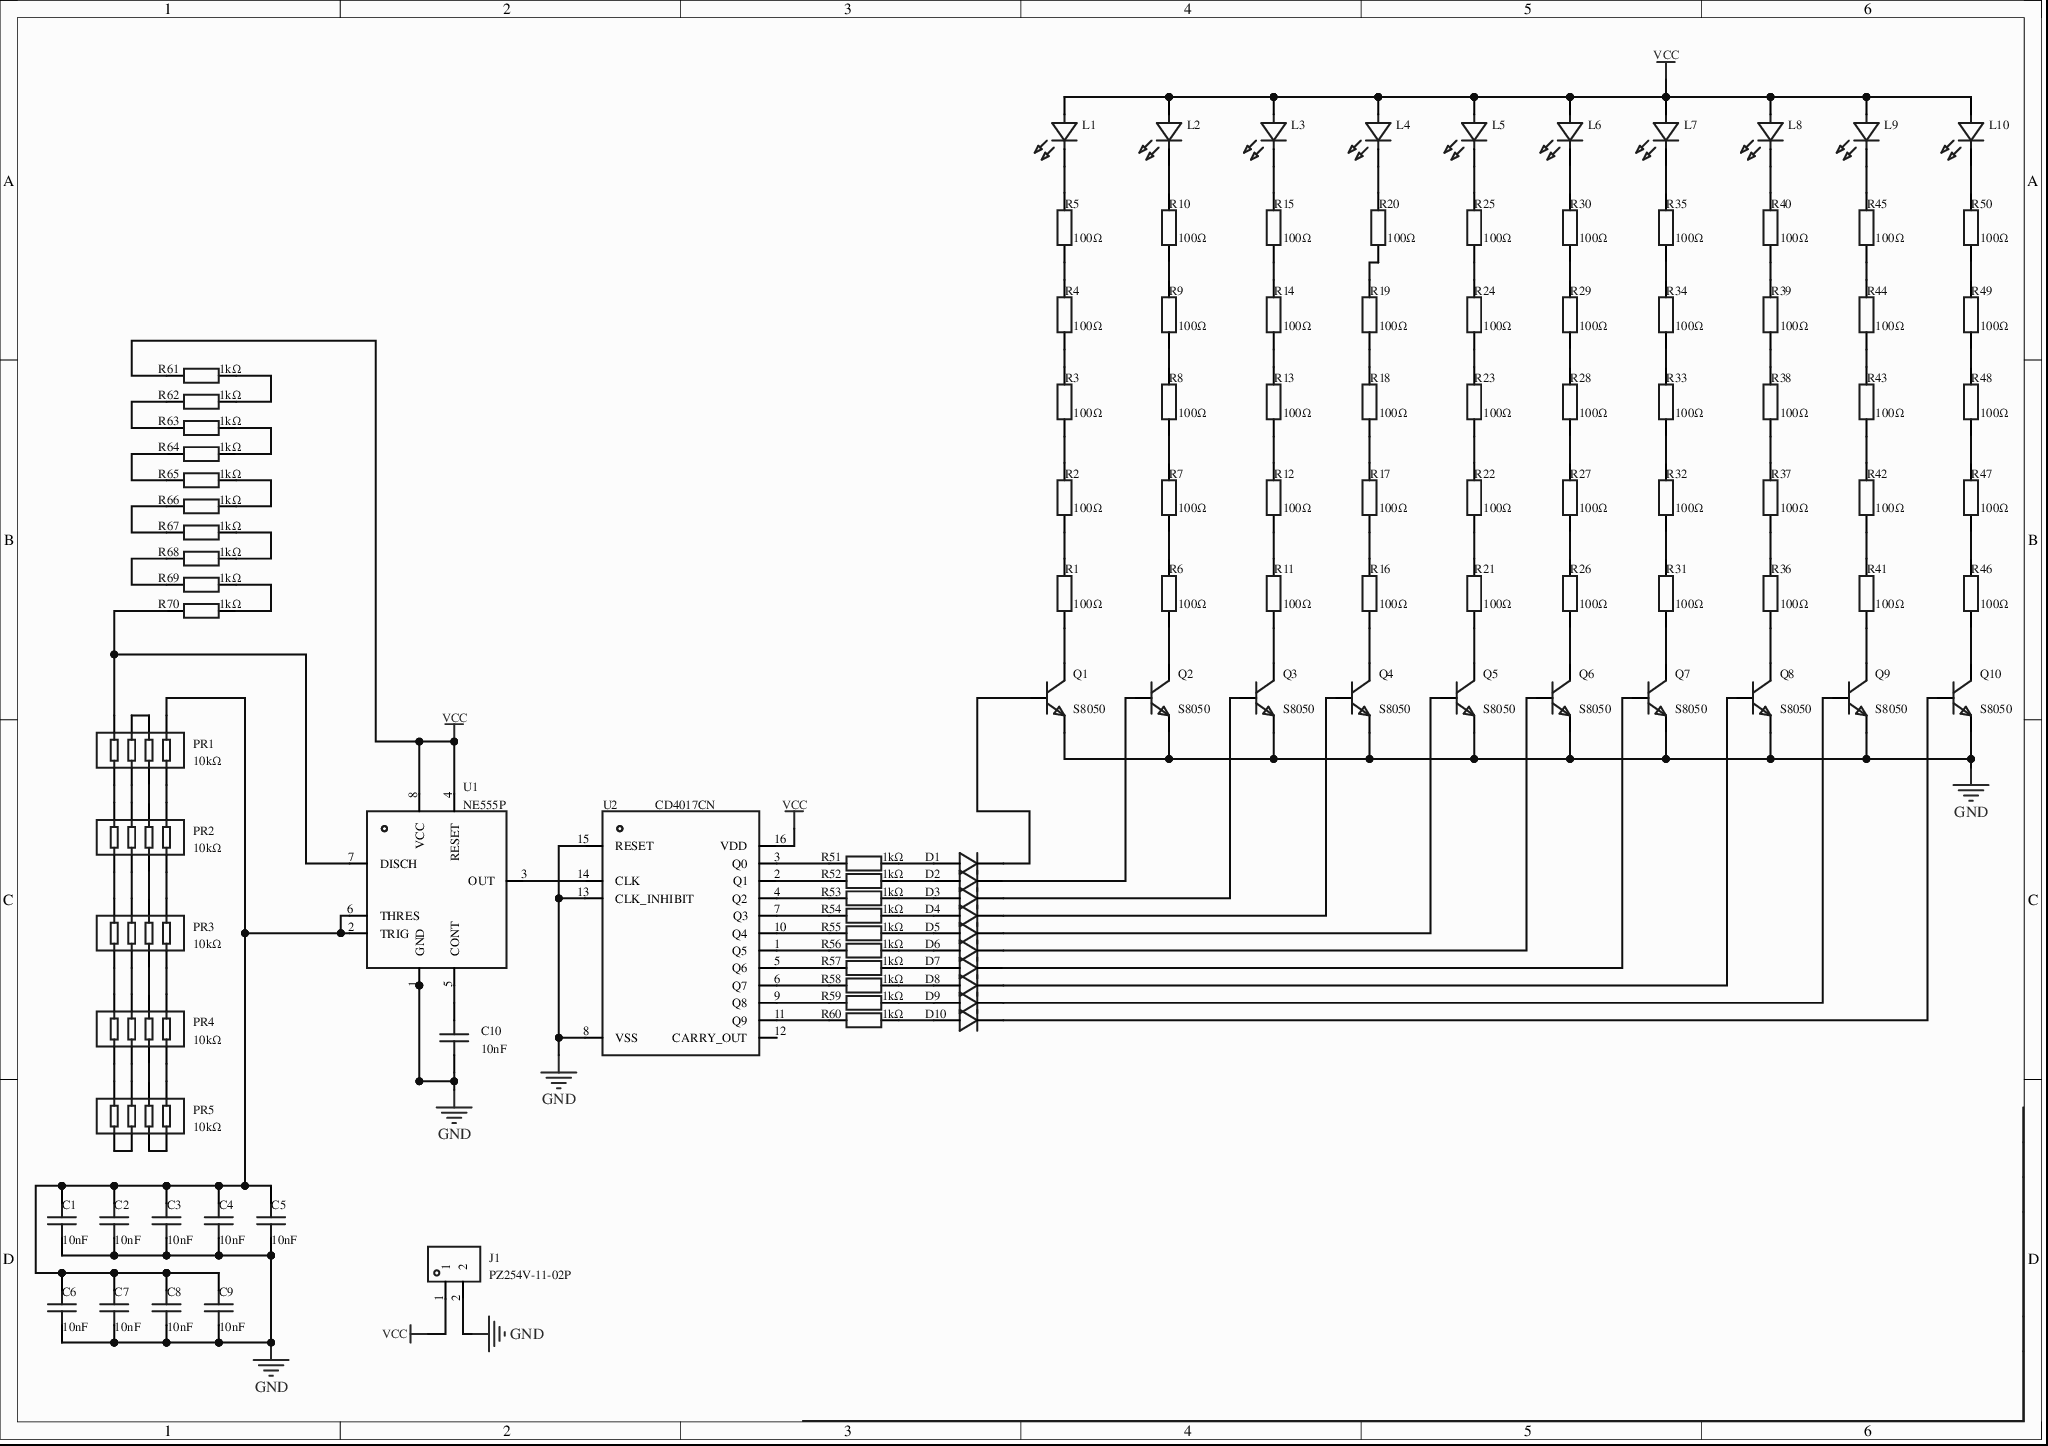
[diagram p0: MISC51825-3.schdoc]
# Altium project MISC51825-2.PrjPcb
1 sheet, 118 parts. Net scope: global (net labels, ports and power ports of the same name join across sheets).
Board file: MISC51825.pcbdoc

## Sheet MISC51825-3.schdoc
size 297 x 209 mm; Version: V1.0; @Project Name: MISC51825; @Page Count: 1; @Update Date: 2026-04-22; @Create Date: 2026-04-22; @Schematic Name: MISC51825; @Page No: 1; @Board Name: MISC51825; @Create Time: 14:32:28; @Update Time: 14:38:12; Size: A4

### Parts
C1  10nF  [CAP-TH_L8.0-W2.8-P5.08-D0.6]
C2  10nF  [CAP-TH_L8.0-W2.8-P5.08-D0.6]
C3  10nF  [CAP-TH_L8.0-W2.8-P5.08-D0.6]
C4  10nF  [CAP-TH_L8.0-W2.8-P5.08-D0.6]
C5  10nF  [CAP-TH_L8.0-W2.8-P5.08-D0.6]
C6  10nF  [CAP-TH_L8.0-W2.8-P5.08-D0.6]
C7  10nF  [CAP-TH_L8.0-W2.8-P5.08-D0.6]
C8  10nF  [CAP-TH_L8.0-W2.8-P5.08-D0.6]
C9  10nF  [CAP-TH_L8.0-W2.8-P5.08-D0.6]
C10  10nF  [CAP-TH_L8.0-W2.8-P5.08-D0.6]
D1  1N4148TR  [DO-35_BD2.0-L4.2-P8.20-D0.5-RD]  (value not drawn)
D2  1N4148TR  [DO-35_BD2.0-L4.2-P8.20-D0.5-RD]  (value not drawn)
D3  1N4148TR  [DO-35_BD2.0-L4.2-P8.20-D0.5-RD]  (value not drawn)
D4  1N4148TR  [DO-35_BD2.0-L4.2-P8.20-D0.5-RD]  (value not drawn)
D5  1N4148TR  [DO-35_BD2.0-L4.2-P8.20-D0.5-RD]  (value not drawn)
D6  1N4148TR  [DO-35_BD2.0-L4.2-P8.20-D0.5-RD]  (value not drawn)
D7  1N4148TR  [DO-35_BD2.0-L4.2-P8.20-D0.5-RD]  (value not drawn)
D8  1N4148TR  [DO-35_BD2.0-L4.2-P8.20-D0.5-RD]  (value not drawn)
D9  1N4148TR  [DO-35_BD2.0-L4.2-P8.20-D0.5-RD]  (value not drawn)
D10  1N4148TR  [DO-35_BD2.0-L4.2-P8.20-D0.5-RD]  (value not drawn)
J1  PZ254V-11-02P  [HDR-TH_2P-P2.54-V-M]
L1  XL-502SURD  [LED-TH_BD5.9-P2.54-RD_RED]  (value not drawn)
L2  XL-502SURD  [LED-TH_BD5.9-P2.54-RD_RED]  (value not drawn)
L3  XL-502SURD  [LED-TH_BD5.9-P2.54-RD_RED]  (value not drawn)
L4  XL-502SURD  [LED-TH_BD5.9-P2.54-RD_RED]  (value not drawn)
L5  XL-502SURD  [LED-TH_BD5.9-P2.54-RD_RED]  (value not drawn)
L6  XL-502SURD  [LED-TH_BD5.9-P2.54-RD_RED]  (value not drawn)
L7  XL-502SURD  [LED-TH_BD5.9-P2.54-RD_RED]  (value not drawn)
L8  XL-502SURD  [LED-TH_BD5.9-P2.54-RD_RED]  (value not drawn)
L9  XL-502SURD  [LED-TH_BD5.9-P2.54-RD_RED]  (value not drawn)
L10  XL-502SURD  [LED-TH_BD5.9-P2.54-RD_RED]  (value not drawn)
PR1  10kΩ  [RES-ARRAY-TH_8P-L20.3-W2.5-P2.54]
PR2  10kΩ  [RES-ARRAY-TH_8P-L20.3-W2.5-P2.54]
PR3  10kΩ  [RES-ARRAY-TH_8P-L20.3-W2.5-P2.54]
PR4  10kΩ  [RES-ARRAY-TH_8P-L20.3-W2.5-P2.54]
PR5  10kΩ  [RES-ARRAY-TH_8P-L20.3-W2.5-P2.54]
Q1  S8050  [TO-92-3_L4.5-W3.5-P1.27-L]
Q2  S8050  [TO-92-3_L4.5-W3.5-P1.27-L]
Q3  S8050  [TO-92-3_L4.5-W3.5-P1.27-L]
Q4  S8050  [TO-92-3_L4.5-W3.5-P1.27-L]
Q5  S8050  [TO-92-3_L4.5-W3.5-P1.27-L]
Q6  S8050  [TO-92-3_L4.5-W3.5-P1.27-L]
Q7  S8050  [TO-92-3_L4.5-W3.5-P1.27-L]
Q8  S8050  [TO-92-3_L4.5-W3.5-P1.27-L]
Q9  S8050  [TO-92-3_L4.5-W3.5-P1.27-L]
Q10  S8050  [TO-92-3_L4.5-W3.5-P1.27-L]
R1  100Ω  [RES-TH_BD2.2-L6.5-P10.50-D0.6]
R2  100Ω  [RES-TH_BD2.2-L6.5-P10.50-D0.6]
R3  100Ω  [RES-TH_BD2.2-L6.5-P10.50-D0.6]
R4  100Ω  [RES-TH_BD2.2-L6.5-P10.50-D0.6]
R5  100Ω  [RES-TH_BD2.2-L6.5-P10.50-D0.6]
R6  100Ω  [RES-TH_BD2.2-L6.5-P10.50-D0.6]
R7  100Ω  [RES-TH_BD2.2-L6.5-P10.50-D0.6]
R8  100Ω  [RES-TH_BD2.2-L6.5-P10.50-D0.6]
R9  100Ω  [RES-TH_BD2.2-L6.5-P10.50-D0.6]
R10  100Ω  [RES-TH_BD2.2-L6.5-P10.50-D0.6]
R11  100Ω  [RES-TH_BD2.2-L6.5-P10.50-D0.6]
R12  100Ω  [RES-TH_BD2.2-L6.5-P10.50-D0.6]
R13  100Ω  [RES-TH_BD2.2-L6.5-P10.50-D0.6]
R14  100Ω  [RES-TH_BD2.2-L6.5-P10.50-D0.6]
R15  100Ω  [RES-TH_BD2.2-L6.5-P10.50-D0.6]
R16  100Ω  [RES-TH_BD2.2-L6.5-P10.50-D0.6]
R17  100Ω  [RES-TH_BD2.2-L6.5-P10.50-D0.6]
R18  100Ω  [RES-TH_BD2.2-L6.5-P10.50-D0.6]
R19  100Ω  [RES-TH_BD2.2-L6.5-P10.50-D0.6]
R20  100Ω  [RES-TH_BD2.2-L6.5-P10.50-D0.6]
R21  100Ω  [RES-TH_BD2.2-L6.5-P10.50-D0.6]
R22  100Ω  [RES-TH_BD2.2-L6.5-P10.50-D0.6]
R23  100Ω  [RES-TH_BD2.2-L6.5-P10.50-D0.6]
R24  100Ω  [RES-TH_BD2.2-L6.5-P10.50-D0.6]
R25  100Ω  [RES-TH_BD2.2-L6.5-P10.50-D0.6]
R26  100Ω  [RES-TH_BD2.2-L6.5-P10.50-D0.6]
R27  100Ω  [RES-TH_BD2.2-L6.5-P10.50-D0.6]
R28  100Ω  [RES-TH_BD2.2-L6.5-P10.50-D0.6]
R29  100Ω  [RES-TH_BD2.2-L6.5-P10.50-D0.6]
R30  100Ω  [RES-TH_BD2.2-L6.5-P10.50-D0.6]
R31  100Ω  [RES-TH_BD2.2-L6.5-P10.50-D0.6]
R32  100Ω  [RES-TH_BD2.2-L6.5-P10.50-D0.6]
R33  100Ω  [RES-TH_BD2.2-L6.5-P10.50-D0.6]
R34  100Ω  [RES-TH_BD2.2-L6.5-P10.50-D0.6]
R35  100Ω  [RES-TH_BD2.2-L6.5-P10.50-D0.6]
R36  100Ω  [RES-TH_BD2.2-L6.5-P10.50-D0.6]
R37  100Ω  [RES-TH_BD2.2-L6.5-P10.50-D0.6]
R38  100Ω  [RES-TH_BD2.2-L6.5-P10.50-D0.6]
R39  100Ω  [RES-TH_BD2.2-L6.5-P10.50-D0.6]
R40  100Ω  [RES-TH_BD2.2-L6.5-P10.50-D0.6]
R41  100Ω  [RES-TH_BD2.2-L6.5-P10.50-D0.6]
R42  100Ω  [RES-TH_BD2.2-L6.5-P10.50-D0.6]
R43  100Ω  [RES-TH_BD2.2-L6.5-P10.50-D0.6]
R44  100Ω  [RES-TH_BD2.2-L6.5-P10.50-D0.6]
R45  100Ω  [RES-TH_BD2.2-L6.5-P10.50-D0.6]
R46  100Ω  [RES-TH_BD2.2-L6.5-P10.50-D0.6]
R47  100Ω  [RES-TH_BD2.2-L6.5-P10.50-D0.6]
R48  100Ω  [RES-TH_BD2.2-L6.5-P10.50-D0.6]
R49  100Ω  [RES-TH_BD2.2-L6.5-P10.50-D0.6]
R50  100Ω  [RES-TH_BD2.2-L6.5-P10.50-D0.6]
R51  1kΩ  [RES-TH_BD2.5-L6.5-P10.50-D0.6]
R52  1kΩ  [RES-TH_BD2.5-L6.5-P10.50-D0.6]
R53  1kΩ  [RES-TH_BD2.5-L6.5-P10.50-D0.6]
R54  1kΩ  [RES-TH_BD2.5-L6.5-P10.50-D0.6]
R55  1kΩ  [RES-TH_BD2.5-L6.5-P10.50-D0.6]
R56  1kΩ  [RES-TH_BD2.5-L6.5-P10.50-D0.6]
R57  1kΩ  [RES-TH_BD2.5-L6.5-P10.50-D0.6]
R58  1kΩ  [RES-TH_BD2.5-L6.5-P10.50-D0.6]
R59  1kΩ  [RES-TH_BD2.5-L6.5-P10.50-D0.6]
R60  1kΩ  [RES-TH_BD2.5-L6.5-P10.50-D0.6]
R61  1kΩ  [RES-TH_BD2.5-L6.5-P10.50-D0.6]
R62  1kΩ  [RES-TH_BD2.5-L6.5-P10.50-D0.6]
R63  1kΩ  [RES-TH_BD2.5-L6.5-P10.50-D0.6]
R64  1kΩ  [RES-TH_BD2.5-L6.5-P10.50-D0.6]
R65  1kΩ  [RES-TH_BD2.5-L6.5-P10.50-D0.6]
R66  1kΩ  [RES-TH_BD2.5-L6.5-P10.50-D0.6]
R67  1kΩ  [RES-TH_BD2.5-L6.5-P10.50-D0.6]
R68  1kΩ  [RES-TH_BD2.5-L6.5-P10.50-D0.6]
R69  1kΩ  [RES-TH_BD2.5-L6.5-P10.50-D0.6]
R70  1kΩ  [RES-TH_BD2.5-L6.5-P10.50-D0.6]
U1  NE555P  [DIP-8_L9.8-W6.6-P2.54-LS7.6-BL]
U2  CD4017CN  [PDIP-16_L19.3-W6.4-P2.54-LS7.94-BL]

### Nets
GND: C1.1 C2.1 C3.1 C4.1 C5.1 C6.1 C7.1 C8.1 C9.1 C10.1 J1.2 Q1.1(E) Q2.1(E) Q3.1(E) Q4.1(E) Q5.1(E) Q6.1(E) Q7.1(E) Q8.1(E) Q9.1(E) Q10.1(E) U1.1(GND) U2.8(VSS) U2.13(CLK_INHIBIT) U2.15(RESET)
VCC: J1.1 L1.2(A) L2.2(A) L3.2(A) L4.2(A) L5.2(A) L6.2(A) L7.2(A) L8.2(A) L9.2(A) L10.2(A) R61.1 U1.4(RESET) U1.8(VCC) U2.16(VDD)
NetC1_2: C1.2 C2.2 C3.2 C4.2 C5.2 C6.2 C7.2 C8.2 C9.2 PR1.5 U1.2(TRIG) U1.6(THRES)
NetC10_2: C10.2 U1.5(CONT)
NetD1_1: D1.1(C) Q1.2(B)
NetD1_2: D1.2(A) R51.2
NetD2_1: D2.1(C) Q2.2(B)
NetD2_2: D2.2(A) R52.2
NetD3_1: D3.1(C) Q3.2(B)
NetD3_2: D3.2(A) R53.2
NetD4_1: D4.1(C) Q4.2(B)
NetD4_2: D4.2(A) R54.2
NetD5_1: D5.1(C) Q5.2(B)
NetD5_2: D5.2(A) R55.2
NetD6_1: D6.1(C) Q6.2(B)
NetD6_2: D6.2(A) R56.2
NetD7_1: D7.1(C) Q7.2(B)
NetD7_2: D7.2(A) R57.2
NetD8_1: D8.1(C) Q8.2(B)
NetD8_2: D8.2(A) R58.2
NetD9_1: D9.1(C) Q9.2(B)
NetD9_2: D9.2(A) R59.2
NetD10_1: D10.1(C) Q10.2(B)
NetD10_2: D10.2(A) R60.2
NetL1_1: L1.1(K) R5.2
NetL2_1: L2.1(K) R10.2
NetL3_1: L3.1(K) R15.2
NetL4_1: L4.1(K) R20.2
NetL5_1: L5.1(K) R25.2
NetL6_1: L6.1(K) R30.2
NetL7_1: L7.1(K) R35.2
NetL8_1: L8.1(K) R40.2
NetL9_1: L9.1(K) R45.2
NetL10_1: L10.1(K) R50.2
NetPR1_1: PR1.1 PR2.8
NetPR1_2: PR1.2 PR2.7
NetPR1_3: PR1.3 PR2.6
NetPR1_4: PR1.4 PR2.5
NetPR1_6: PR1.6 PR1.7
NetPR1_8: PR1.8 R70.1 U1.7(DISCH)
NetPR2_1: PR2.1 PR3.8
NetPR2_2: PR2.2 PR3.7
NetPR2_3: PR2.3 PR3.6
NetPR2_4: PR2.4 PR3.5
NetPR3_1: PR3.1 PR4.8
NetPR3_2: PR3.2 PR4.7
NetPR3_3: PR3.3 PR4.6
NetPR3_4: PR3.4 PR4.5
NetPR4_1: PR4.1 PR5.8
NetPR4_2: PR4.2 PR5.7
NetPR4_3: PR4.3 PR5.6
NetPR4_4: PR4.4 PR5.5
NetPR5_1: PR5.1 PR5.2
NetPR5_3: PR5.3 PR5.4
NetQ1_3: Q1.3(C) R1.1
NetQ2_3: Q2.3(C) R6.1
NetQ3_3: Q3.3(C) R11.1
NetQ4_3: Q4.3(C) R16.1
NetQ5_3: Q5.3(C) R21.1
NetQ6_3: Q6.3(C) R26.1
NetQ7_3: Q7.3(C) R31.1
NetQ8_3: Q8.3(C) R36.1
NetQ9_3: Q9.3(C) R41.1
NetQ10_3: Q10.3(C) R46.1
NetR1_2: R1.2 R2.1
NetR2_2: R2.2 R3.1
NetR3_2: R3.2 R4.1
NetR4_2: R4.2 R5.1
NetR6_2: R6.2 R7.1
NetR7_2: R7.2 R8.1
NetR8_2: R8.2 R9.1
NetR9_2: R9.2 R10.1
NetR11_2: R11.2 R12.1
NetR12_2: R12.2 R13.1
NetR13_2: R13.2 R14.1
NetR14_2: R14.2 R15.1
NetR16_2: R16.2 R17.1
NetR17_2: R17.2 R18.1
NetR18_2: R18.2 R19.1
NetR19_2: R19.2 R20.1
NetR21_2: R21.2 R22.1
NetR22_2: R22.2 R23.1
NetR23_2: R23.2 R24.1
NetR24_2: R24.2 R25.1
NetR26_2: R26.2 R27.1
NetR27_2: R27.2 R28.1
NetR28_2: R28.2 R29.1
NetR29_2: R29.2 R30.1
NetR31_2: R31.2 R32.1
NetR32_2: R32.2 R33.1
NetR33_2: R33.2 R34.1
NetR34_2: R34.2 R35.1
NetR36_2: R36.2 R37.1
NetR37_2: R37.2 R38.1
NetR38_2: R38.2 R39.1
NetR39_2: R39.2 R40.1
NetR41_2: R41.2 R42.1
NetR42_2: R42.2 R43.1
NetR43_2: R43.2 R44.1
NetR44_2: R44.2 R45.1
NetR46_2: R46.2 R47.1
NetR47_2: R47.2 R48.1
NetR48_2: R48.2 R49.1
NetR49_2: R49.2 R50.1
NetR51_1: R51.1 U2.3(Q0)
NetR52_1: R52.1 U2.2(Q1)
NetR53_1: R53.1 U2.4(Q2)
NetR54_1: R54.1 U2.7(Q3)
NetR55_1: R55.1 U2.10(Q4)
NetR56_1: R56.1 U2.1(Q5)
NetR57_1: R57.1 U2.5(Q6)
NetR58_1: R58.1 U2.6(Q7)
NetR59_1: R59.1 U2.9(Q8)
NetR60_1: R60.1 U2.11(Q9)
NetR61_2: R61.2 R62.2
NetR62_1: R62.1 R63.1
NetR63_2: R63.2 R64.2
NetR64_1: R64.1 R65.1
NetR65_2: R65.2 R66.2
NetR66_1: R66.1 R67.1
NetR67_2: R67.2 R68.2
NetR68_1: R68.1 R69.1
NetR69_2: R69.2 R70.2
NetU1_3: U1.3(OUT) U2.14(CLK)

Not connected (* = marked no-connect by the designer): U2 12(CARRY_OUT)

### Library data of the parts
C1-C10 = CC3A103MC1IEF48C30MF: 容值:10nF;精度:±20%;额定电压:1kV;温度系数:Y5V;; Manufacturer: Dersonic(德尔创); AddInBom: yes; Tolerance: ±20%; Voltage Rating: 1kV; Pin Spacing: 5.08mm; Temperature Coefficient: Y5V; Body Thickness: 2.8mm; ModelId: adc2ba9dad3c618c; ModelTransform: 0,0,0,0,0,0,0,0,0; Device: CC3A103MC1IEF48C30MF; Symbol: CC3A103MC1IEF48C30MF; FootprintName: CAP-TH_L8.0-W2.8-P5.08-D0.6; LCSC Part Name: 10nF ±20% 1kV; SupplierPart: C263209; ManufacturerPart: CC3A103MC1IEF48C30MF; Supplier Footprint: 插件,P=5.08mm; JLCPCB Part Class: 扩展库; Datasheet: https://item.szlcsc.com/datasheet/CC3A103MC1IEF48C30MF/254325.html; Supplier: LCSC; ConvertToPcb: yes; Value: 10nF; Diameter: 8mm; ModelName: CAP-TH_L8.0-W2.8-P5.08-D0.6
D1-D10 = 1N4148TR_C84410: 二极管配置:-;正向压降(Vf):1V@10mA;直流反向耐压(Vr):100V;整流电流:200mA;反向恢复时间(Trr):4ns;; Manufacturer: onsemi(安森美); AddInBom: yes; Voltage - DC Reverse(Vr): 100V; Current - Rectified: 200mA; Pd - Power Dissipation: 500mW; Reverse Leakage Current (Ir): 5uA@75V; Reverse Recovery Time (trr): 4ns; Operating Junction Temperature Range: -55℃~+175℃@(Tj); Non-Repetitive Peak Forward Surge Current: 4A; ModelId: 6e6fa891745c42b796728c269d94cdcf; ModelName: DO-35_D1.9-L3.9-P8.2; ModelTransform: 342.519,74.82103,0,0,0,0,-0.197,1.181,-137.795; Device: 1N4148TR_C84410; Symbol: 1N4148TR; FootprintName: DO-35_BD2.0-L4.2-P8.20-D0.5-RD; LCSC Part Name: 1N4148TR; SupplierPart: C84410; ManufacturerPart: 1N4148TR; Supplier Footprint: DO-35; JLCPCB Part Class: 扩展库; Datasheet: https://item.szlcsc.com/datasheet/1N4148TR/85580.html; Supplier: LCSC; ConvertToPcb: yes; Diode Configuration: -; Voltage - Forward(Vf@If): 1V@10mA
J1 = PZ254V-11-02P: 插针结构:1x2P;间距:2.54mm;行距:-;圆针/方针:方针;安装方式:直插;排数:单排;总PIN位数:2P;额定电流:3A;额定电压:250V;配合针长度:6mm;塑高:2.5mm;端接针长度:3mm;触头材质:黄铜;触头镀层:-;工作温度:-40℃~+105℃;颜色:黑色;; Manufacturer: XFCN(兴飞); AddInBom: yes; Pin Structure: 1x2P; Pitch: 2.54mm; Circluar Pins/Square Pins: 方针; Current Rating: 3A; Voltage Rating (Max): 250V; ModelId: e35305ec3aa84b66b849f914b715e73f; ModelName: HDR2.54-M-LI-1X2P; ModelTransform: 200,100,0,0,0,0,0,0,-118.11; Device: PZ254V-11-02P; Symbol: PZ254V-11-02P; FootprintName: HDR-TH_2P-P2.54-V-M; LCSC Part Name: 1x2P 间距:2.54mm 方针 直插; SupplierPart: C492401; ManufacturerPart: PZ254V-11-02P; Supplier Footprint: 插件,P=2.54mm; JLCPCB Part Class: 扩展库; Datasheet: https://item.szlcsc.com/datasheet/PZ254V-11-02P/502957.html; Supplier: LCSC; ConvertToPcb: yes; Row Spacing: -; Mounting Type: 直插; Number of Rows: 单排; Number of Pins: 2P; Length of Mating Pin: 6mm; Insulation Height: 2.5mm; Length of End Connection Pin: 3mm; Contact Material: 黄铜; Contact Plating: -; Operating Temperature: -40℃~+105℃; Color: 黑色
L1-L10 = XL-502SURD: 灯头类型:5mm圆形灯头;发光颜色:红色;正向压降(Vf):2.4V;功率:70mW;正向电流:20mA;波长:615nm~625nm;二极管配置:-;透镜颜色:红色透镜;色温:-;发光强度:300mcd;发光角度:35°;载带方式:-;工作温度:-25℃~+85℃;; Manufacturer: XINGLIGHT(成兴光); AddInBom: yes; Illumination Color: 红色; Voltage - Forward(Vf): 2.4V; Power(Watts): 70mW; Forward Current: 20mA; Peak Wavelength: 654nm; Lens Color: 红色透镜; Luminous Intensity: 300mcd; Viewing Angle: 35°; ModelId: fe9cea1bdf7642cd8d9a5077ed0e2b58; ModelTransform: 211.96686,228.01584,0,0,0,0,7.874,0,-137.795; Device: XL-502SURD; Symbol: XL-502SURD; FootprintName: LED-TH_BD5.9-P2.54-RD_RED; LCSC Part Name: 5mm圆形灯头 红色; SupplierPart: C2895492; ManufacturerPart: XL-502SURD; Supplier Footprint: 插件,D=5mm; JLCPCB Part Class: 扩展库; Datasheet: https://item.szlcsc.com/datasheet/XL-502SURD/3136207.html; Supplier: LCSC; ConvertToPcb: yes; Lamp Holder Type: 5mm圆形灯头; Wavelength - Dominant: 615nm~625nm; Diode Configuration: -; Color Temperature: -; Mounting Style: -; Operating Temperature: -25℃~+85℃; ModelName: LED-TH_BD5.9-P2.54-RD_RED
PR1-PR5 = 4608X-102-103LF: 电阻器数:4;阻值:10kΩ;精度:±2%;单个元件功率:300mW;温度系数:±100ppm/℃;; Manufacturer: BOURNS; AddInBom: yes; Number of Resistors: 4; Tolerance: ±2%; Power(Watts): 300mW; ModelId: 1fcaf8e202754517bf5022a866f874ea; ModelTransform: 798.02982,98.031,0,0,0,0,0,0,-133.858; Device: 4608X-102-103LF; Symbol: 4608X-102-103LF; FootprintName: RES-ARRAY-TH_8P-L20.3-W2.5-P2.54; LCSC Part Name: 10kΩ ±2%; SupplierPart: C840662; ManufacturerPart: 4608X-102-103LF; Supplier Footprint: SIP-8; JLCPCB Part Class: 扩展库; Datasheet: https://item.szlcsc.com/datasheet/4608X-102-103LF/897114.html; Supplier: LCSC; ConvertToPcb: yes; Value: 10kΩ; Temperature Coefficient: ±100ppm/℃; Number of Pins: 8; ModelName: RES-ARRAY-TH_8P-L20.3-W2.5-P2.54
Q1-Q10 = S8050_C2931492: 晶体管类型:NPN;集电极电流(Ic):500mA;集射极击穿电压(Vceo):25V;耗散功率(Pd):625mW;直流电流增益(hFE):160@50mA,1V;; Manufacturer: JSMSEMI(杰盛微); AddInBom: yes; type: NPN; Current - Collector(Ic): 500mA; Collector - Emitter Voltage VCEO: 25V; Pd - Power Dissipation: 625mW; Transition frequency(fT): 150MHz; Current - Collector Cutoff: 100nA; Vce Saturation(VCE(sat)): 600mV@500mA,50mA; Emitter-Base Voltage(Vebo): 5V; ModelId: 3c10f07c6cc72ff5; ModelTransform: 0,0,0,0,0,0,0,0,0; Device: S8050_C2931492; Symbol: S8050_C2931492; FootprintName: TO-92-3_L4.5-W3.5-P1.27-L; LCSC Part Name: NPN 电流:500mA 电压:25V; SupplierPart: C2931492; ManufacturerPart: S8050; Supplier Footprint: TO-92; JLCPCB Part Class: 扩展库; Datasheet: https://item.szlcsc.com/datasheet/S8050/3272796.html; Supplier: LCSC; ConvertToPcb: yes; DC Current Gain: 160@50mA,1V; ModelName: TO-92-3_L4.5-W3.5-P1.27-L
R1-R50 = MFR0W4F1000A50: 电阻类型:金属膜电阻;阻值:100Ω;精度:±1%;功率:250mW;温度系数:±50ppm/℃;; Manufacturer: UNI-ROYAL(厚声); AddInBom: yes; Tolerance: ±1%; Voltage-Supply(Max): 250V; Power(Watts): 250mW; ModelId: 094322567e2be2d4; ModelTransform: 0,0,0,0,0,0,0,0,0; Device: MFR0W4F1000A50; Symbol: MFR0W4F1000A50; FootprintName: RES-TH_BD2.2-L6.5-P10.50-D0.6; LCSC Part Name: 100Ω ±1% 250mW 金属膜电阻 铜脚，圆柱状直插; SupplierPart: C57438; ManufacturerPart: MFR0W4F1000A50; Supplier Footprint: 插件,D2.2xL6.5mm; JLCPCB Part Class: 扩展库; Datasheet: https://atta.szlcsc.com/upload/public/pdf/source/20191012/C436293_8820AA14BC71FA35E551C06C441482A0.pdf; Supplier: LCSC; ConvertToPcb: yes; Type: 金属膜电阻; Value: 100Ω; Temperature Coefficient: ±50ppm/℃; ModelName: RES-TH_BD2.2-L6.5-P10.50-D0.6
R51-R70 = MFR0W4F1001A50: 电阻类型:金属膜电阻;阻值:1kΩ;精度:±1%;功率:250mW;温度系数:±50ppm/℃;; Manufacturer: UNI-ROYAL(厚声); AddInBom: yes; Tolerance: ±1%; Voltage-Supply(Max): 250V; Power(Watts): 250mW; ModelId: 8e6c7ee8323443d1ab8f0504b6353c8c; ModelName: RES-TH_D2.3-L6.5-P10.50; ModelTransform: 431.1015,91.3384,0,0,0,0,0.197,0,-137.795; Device: MFR0W4F1001A50; Symbol: MFR0W4F1001A50; FootprintName: RES-TH_BD2.5-L6.5-P10.50-D0.6; LCSC Part Name: 1kΩ ±1% 250mW 金属膜电阻 铜脚，圆柱状直插; SupplierPart: C57435; ManufacturerPart: MFR0W4F1001A50; Supplier Footprint: 插件,D2.2xL6.5mm; JLCPCB Part Class: 扩展库; Datasheet: https://atta.szlcsc.com/upload/public/pdf/source/20191012/C436293_8820AA14BC71FA35E551C06C441482A0.pdf; Supplier: LCSC; ConvertToPcb: yes; Type: 金属膜电阻; Value: 1kΩ; Temperature Coefficient: ±50ppm/℃
U1 = NE555P: 这些器件是精密定时电路，能够产生精确的时间延迟或振荡。在延时或单稳态工作模式下，定时时间间隔由单个外部电阻和电容网络控制。在无稳态工作模式下，频率和占空比可通过两个外部电阻和一个外部电容分别控制; Manufacturer: TI(德州仪器); AddInBom: yes; ModelId: db2af726fcec488f8bf8e467aca974b3; ModelName: DIP-8_L9.8-W6.6-H3.5-LS7.62-P2.54; ModelTransform: 385.826,311.8104,0,0,0,0,-1.693,0,-137.795; Device: NE555P; Symbol: NE555P; FootprintName: DIP-8_L9.8-W6.6-P2.54-LS7.6-BL; LCSC Part Name: NE555P; SupplierPart: C46749; ManufacturerPart: NE555P; Supplier Footprint: DIP-8; JLCPCB Part Class: Extended Part; Datasheet: https://www.ti.com/cn/lit/gpn/ne555; Supplier: LCSC; ConvertToPcb: yes
U2 = CD4017CN: CD4017BE升级替代料，建议试样，5 阶 Johnson 译码计数器; Manufacturer: HGSEMI(华冠); AddInBom: yes; ModelId: 96ff5d01b3074dd183bcbc4cd00a63de; ModelTransform: 759.841,322.44,0,0,0,0,0,0,-137.795; Device: CD4017CN; Symbol: CD4017CN; FootprintName: PDIP-16_L19.3-W6.4-P2.54-LS7.94-BL; LCSC Part Name: CD4017CN; SupplierPart: C20613262; ManufacturerPart: CD4017CN; Supplier Footprint: DIP-16; JLCPCB Part Class: 扩展库; Datasheet: https://atta.szlcsc.com/upload/public/pdf/source/20240202/A11F5FEC5EC92025B33B6A151300674C.pdf; Supplier: LCSC; ConvertToPcb: yes; ModelName: PDIP-16_L19.3-W6.4-P2.54-LS7.94-BL